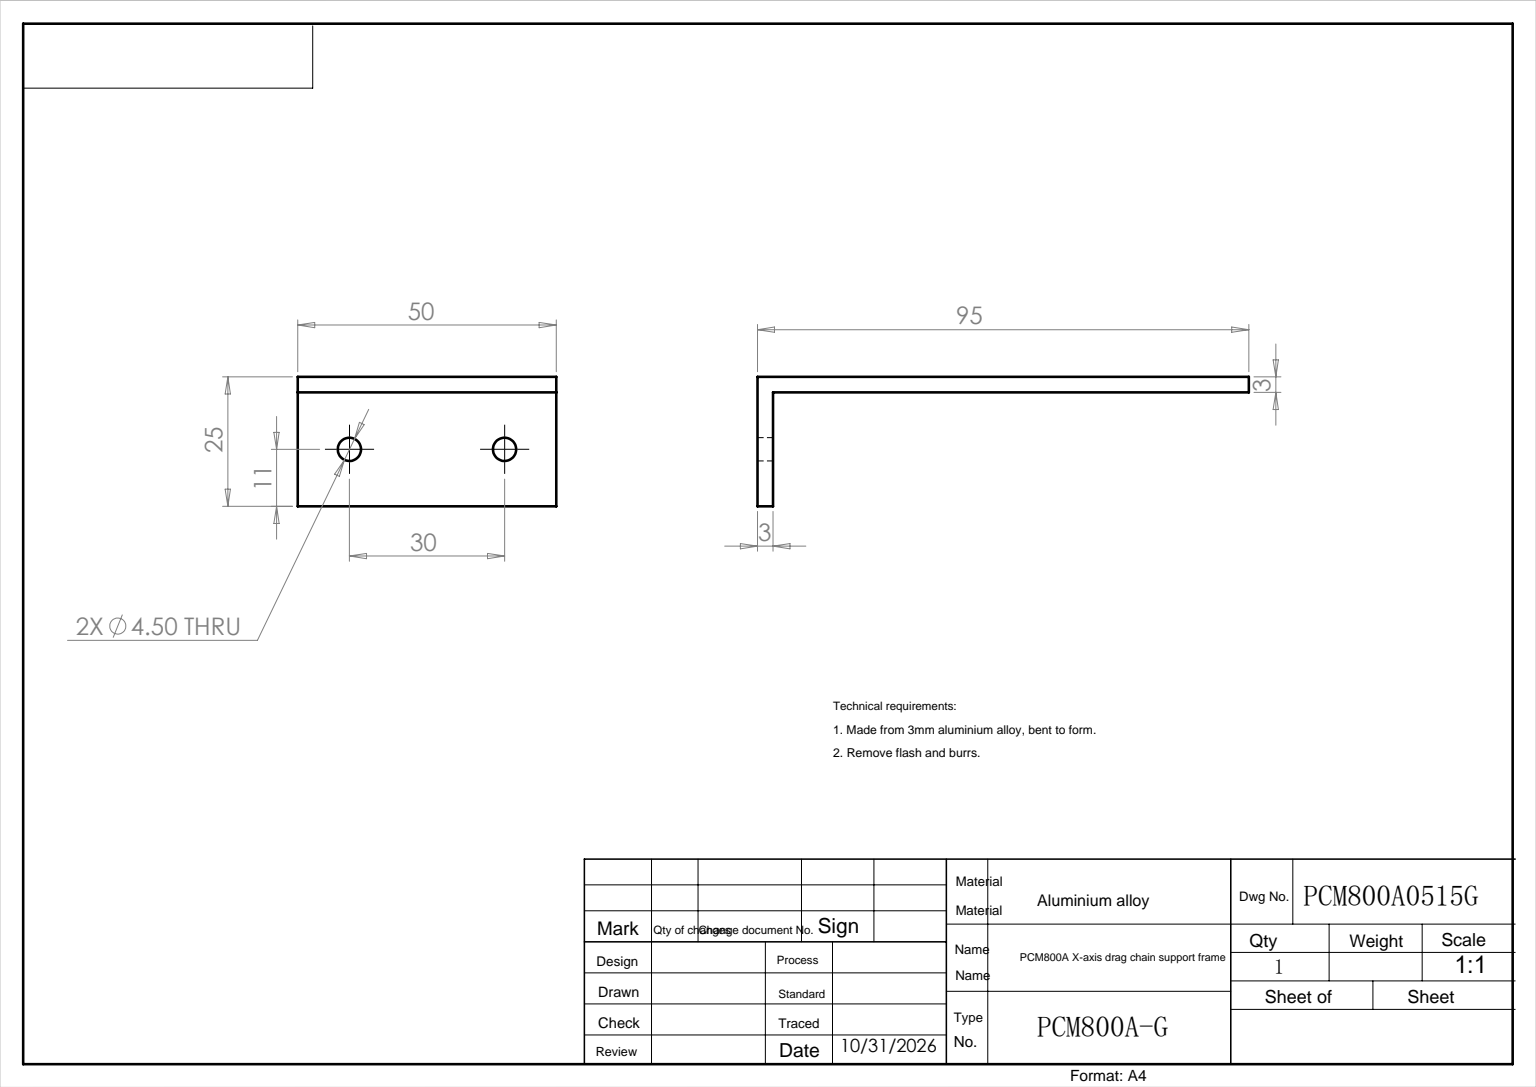
SolidWorks part; units mm, degrees
ref_plane "前视基准面" through (0, 0, 0) normal (0, 0, 1) x (1, 0, 0)
ref_plane "上视基准面" through (0, 0, 0) normal (0, 1, 0) x (1, 0, 0)
ref_plane "右视基准面" through (0, 0, 0) normal (1, 0, 0) x (0, 0, -1)
sketch "草图1" plane through (0, 0, 0) normal (0, 0, 1) x (1, 0, 0)
  line L0 (0, 0) -> (0, 25)
  line L1 (0, 25) -> (95, 25)
  dimension "D1" = 25
  dimension "D2" = 95
extrude "拉伸-薄壁1" add sketch "草图1" along normal blind 50 thin
sketch "草图2" plane through (3, 0, 0) normal (1, 0, 0) x (0, 0, -1)
  line L0 (-50, 11) -> (6.8, 11) construction
  line L1 (-50, 0) -> (-50, 22) construction
  line L2 (-25, 0) -> (-25, 34.124) construction
  line L3 (-50, 0) -> (0, 0) construction
  circle A0 centre (-40, 11) radius 2.25
  circle A1 centre (-10, 11) radius 2.25
  dimension "D1" = 4.5
  dimension "D2" = 15
extrude "切除-拉伸1" cut sketch "草图2" against normal blind 10
